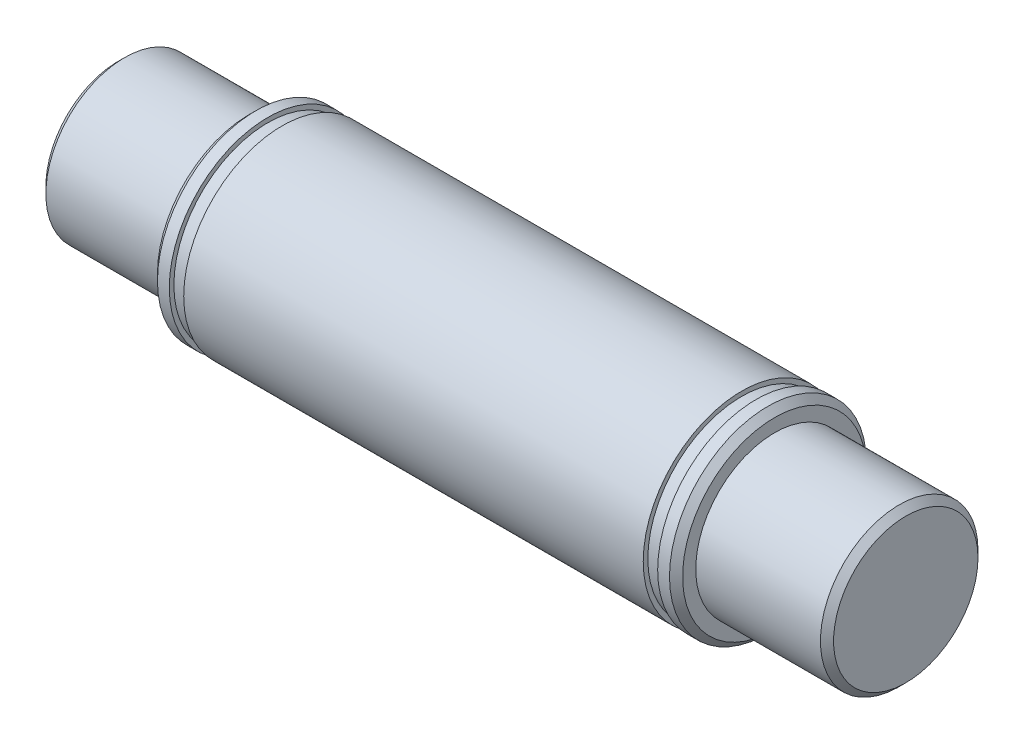
SolidWorks part; units mm, degrees
ref_plane "前视基准面" through (0, 0, 0) normal (0, 0, 1) x (1, 0, 0)
ref_plane "上视基准面" through (0, 0, 0) normal (0, 1, 0) x (1, 0, 0)
ref_plane "右视基准面" through (0, 0, 0) normal (1, 0, 0) x (0, 0, -1)
sketch "草图1" plane through (0, 0, 0) normal (1, 0, 0) x (0, 0, -1)
  circle A0 centre (0, 0) radius 7.5
  dimension "D1" = 15
extrude "凸台-拉伸1" add sketch "草图1" along normal mid plane 60
sketch "草图2" plane through (30, 0, 0) normal (1, 0, 0) x (0, 0, -1)
  circle A0 centre (0, 0) radius 6
  dimension "D1" = 12
extrude "切除-拉伸1" cut sketch "草图2" against normal blind 10 flip side to cut
mirror "镜向1" about plane through (0, 0, 0) normal (1, 0, 0) of "切除-拉伸1"
chamfer "倒角1" distance 0.5 angle 45 4 edges at (30, 0, -6) (20, 0, -7.5) (-20, 0, 7.5) (-30, 0, -6)
sketch "草图3" plane through (0, 0, 0) normal (0, 0, 1) x (1, 0, 0)
  line L0 (-19.5, -7.5) -> (19.5, -7.5) construction
  line L1 (-18.6, -7.5) -> (-17.5, -7.5)
  line L2 (-18.6, -7.5) -> (-18.6, -7.15)
  line L3 (-18.6, -7.15) -> (-17.5, -7.15)
  line L4 (-17.5, -7.5) -> (-17.5, -7.15)
  line L5 (-31.3658, 0) -> (33.4147, 0) construction
  dimension "D1" = 0.35
  dimension "D2" = 1.1
  dimension "D3" = 17.5
revolve "切除-旋转1" cut sketch "草图3" angle 360 about L5
mirror "镜向2" about plane through (0, 0, 0) normal (1, 0, 0) of "切除-旋转1"
